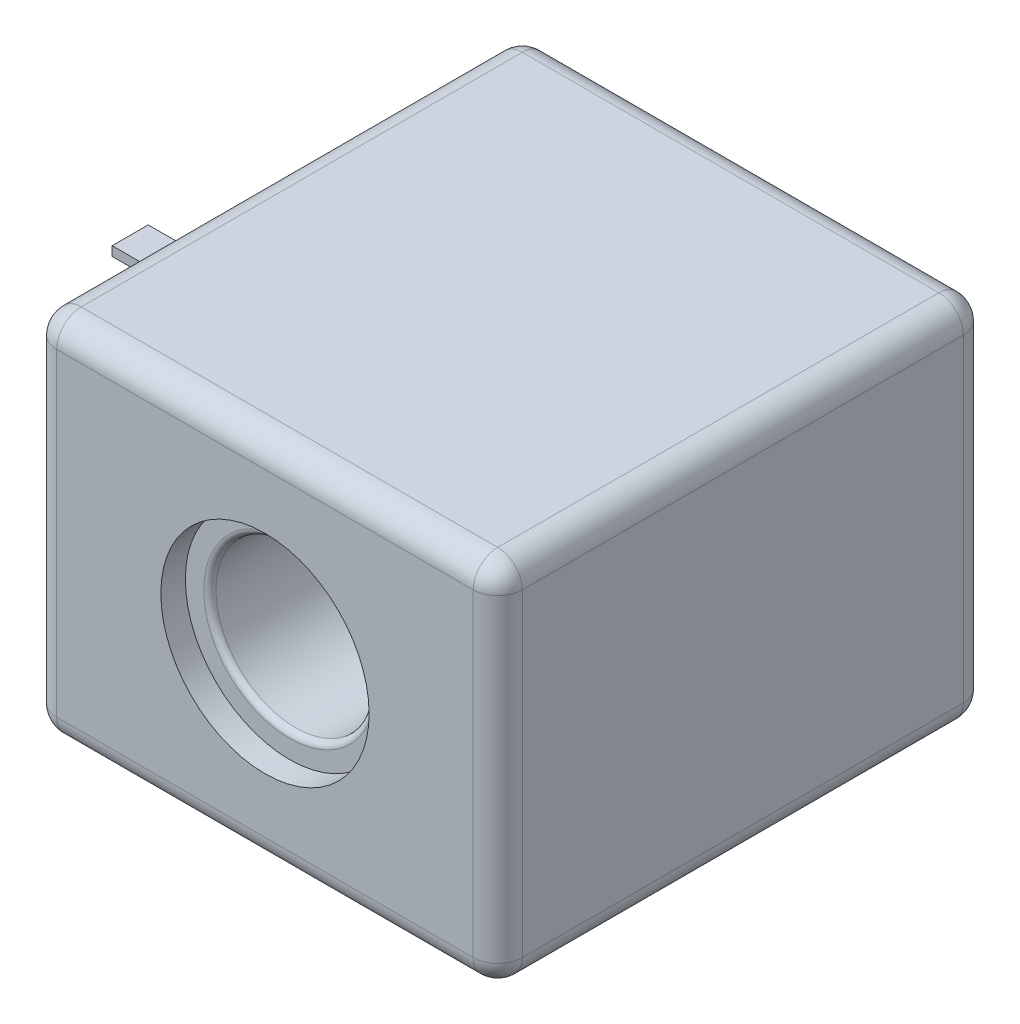
from build123d import *

# Parameters (mm, degrees)
SKETCH1_W           = 38
SKETCH1_H           = 30
BOSS_EXTRUDE1_DEPTH = 40
FILLET1_R           = 2
SKETCH2_R           = 6.5
CUT_EXTRUDE1_DEPTH  = 40
SKETCH3_R           = 8.5
CUT_EXTRUDE2_DEPTH  = 2
CUT_EXTRUDE3_START  = -2
SKETCH4_R           = 8.5
CUT_EXTRUDE3_DEPTH  = 2
FILLET2_R           = 0.5
SKETCH5_R           = 1.5
CUT_EXTRUDE4_DEPTH  = 9
SKETCH6_R           = 2.5
SKETCH6_R_2         = 2.499
CUT_EXTRUDE5_DEPTH  = 9
BOSS_EXTRUDE2_DEPTH = 9
SKETCH8_W           = 0.547536787
SKETCH8_H           = 2.855013248
BOSS_EXTRUDE3_DEPTH = 9


with BuildPart() as part:
    # Sketch1 → Boss-Extrude1 (new body)
    with BuildSketch(Plane.XY):
        Rectangle(SKETCH1_W, SKETCH1_H)
    extrude(amount=BOSS_EXTRUDE1_DEPTH)

    # Fillet1
    fillet1_edges = [part.edges().sort_by_distance(p)[0] for p in [
        (-19, 0, 40),
        (0, -15, 40),
        (19, 0, 40),
        (0, -15, 0),
        (-19, 0, 0),
        (0, 15, 0),
        (19, 0, 0),
        (19, -15, 20),
        (-19, -15, 20),
        (-19, 15, 20),
        (19, 15, 20),
        (0, 15, 40),
    ]]
    fillet(fillet1_edges, radius=FILLET1_R)

    # Sketch2 → Cut-Extrude1 (cut)
    with BuildSketch(Plane.XY.offset(40)):
        Circle(SKETCH2_R)
    extrude(amount=-CUT_EXTRUDE1_DEPTH, mode=Mode.SUBTRACT)

    # Sketch3 → Cut-Extrude2 (cut)
    with BuildSketch(Plane.XY.offset(40)):
        Circle(SKETCH3_R)
    extrude(amount=-CUT_EXTRUDE2_DEPTH, mode=Mode.SUBTRACT)

    # Sketch4 → Cut-Extrude3 (cut)
    with BuildSketch(Plane(origin=(0, 0, 0), x_dir=(-1, 0, 0), z_dir=(0, 0, -1)).offset(CUT_EXTRUDE3_START)):
        with Locations(Location((0, 0, 0), (0, 0, 180))):
            Circle(SKETCH4_R)
    extrude(amount=CUT_EXTRUDE3_DEPTH, mode=Mode.SUBTRACT)

    # Fillet2
    fillet2_edges = [part.edges().sort_by_distance(p)[0] for p in [
        (-6.5, 0, 38),
        (-6.5, 0, 2),
    ]]
    fillet(fillet2_edges, radius=FILLET2_R)

    # Sketch5 → Cut-Extrude4 (cut)
    with BuildSketch(Plane.ZY.offset(19)):
        with Locations(Location((20, 0, 0), (0, 0, 270))):
            Circle(SKETCH5_R)
    extrude(amount=-CUT_EXTRUDE4_DEPTH, mode=Mode.SUBTRACT)

    # Sketch6 → Cut-Extrude5 (cut)
    with BuildSketch(Plane.ZY.offset(19)):
        with Locations(Location((20, 0, 0), (0, 0, 270))):
            Circle(SKETCH6_R)
        with Locations(Location((20, 0, 0), (0, 0, 270))):
            Circle(SKETCH6_R_2, mode=Mode.SUBTRACT)
    extrude(amount=-CUT_EXTRUDE5_DEPTH, mode=Mode.SUBTRACT)

    # Sketch7 → Boss-Extrude2 (add)
    with BuildSketch(Plane.ZY.offset(19)):
        Polygon((21.729521331, -6.29783972), (21.529486226, -6.29783972), (21.529486226, -7.062375907), (24.471577179, -7.062375907), (24.471577179, -6.29783972), (24.271542075, -6.29783972), (24.271542075, -6.708059845), (21.729521331, -6.708059845), align=None)
    boss_extrude2 = extrude(amount=BOSS_EXTRUDE2_DEPTH)

    # Mirror1: Boss-Extrude2 across plane
    add(boss_extrude2.mirror(Plane.ZX))

    # Sketch8 → Boss-Extrude3 (add)
    with BuildSketch(Plane.ZY.offset(19)):
        with Locations((13.819655902, 0.006123147)):
            Rectangle(SKETCH8_W, SKETCH8_H)
    extrude(amount=BOSS_EXTRUDE3_DEPTH)


solid = part.part
